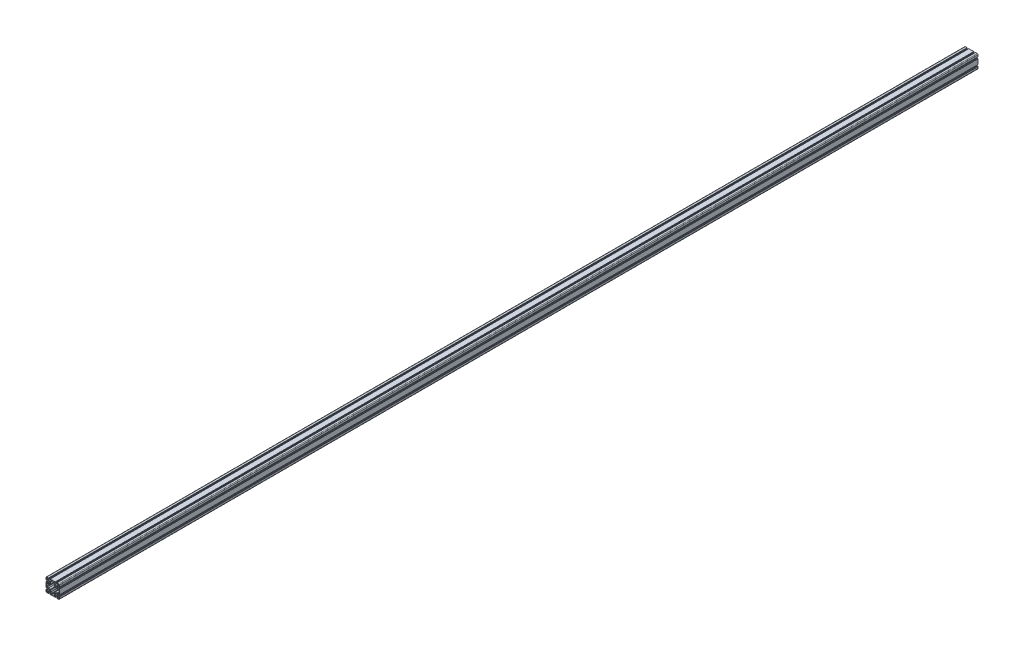
from build123d import *

# Parameters (mm, degrees)
SKETCH1_R           = 3.4
BOSS_EXTRUDE1_DEPTH = 5500


with BuildPart() as part:
    # Sketch1 → Boss-Extrude1 (new body)
    with BuildSketch(Plane.XY.offset(100)):
        with BuildLine():
            Line((37.78472507, 10.370402299), (32.802492023, 10.370402299))
            Line((32.802492023, 10.370402299), (28.48472507, 14.688169252))
            Line((28.48472507, 14.688169252), (28.48472507, 26.552635346))
            Line((28.48472507, 26.552635346), (32.802492023, 30.870402299))
            Line((32.802492023, 30.870402299), (37.78472507, 30.870402299))
            ThreePointArc((37.78472507, 30.870402299), (38.491831851, 30.57750908), (38.78472507, 29.870402299))
            Line((38.78472507, 29.870402299), (38.78472507, 28.220402299))
            ThreePointArc((38.78472507, 28.220402299), (38.491831851, 27.513295518), (37.78472507, 27.220402299))
            Line((37.78472507, 27.220402299), (36.28472507, 27.220402299))
            Line((36.28472507, 27.220402299), (36.28472507, 25.020402299))
            ThreePointArc((36.28472507, 25.020402299), (36.372593036, 24.808270264), (36.58472507, 24.720402299))
            Line((36.58472507, 24.720402299), (39.78472507, 24.720402299))
            Line((39.78472507, 24.720402299), (39.78472507, 25.520402299))
            ThreePointArc((39.78472507, 25.520402299), (39.843303714, 25.661823655), (39.98472507, 25.720402299))
            Line((39.98472507, 25.720402299), (40.78472507, 25.720402299))
            Line((40.78472507, 25.720402299), (40.78472507, 36.120402299))
            ThreePointArc((40.78472507, 36.120402299), (39.466705585, 39.302382814), (36.28472507, 40.620402299))
            Line((36.28472507, 40.620402299), (25.88472507, 40.620402299))
            Line((25.88472507, 40.620402299), (25.88472507, 39.820402299))
            ThreePointArc((25.88472507, 39.820402299), (25.826146426, 39.678980943), (25.68472507, 39.620402299))
            Line((25.68472507, 39.620402299), (24.88472507, 39.620402299))
            Line((24.88472507, 39.620402299), (24.88472507, 36.420402299))
            ThreePointArc((24.88472507, 36.420402299), (24.972593036, 36.208270264), (25.18472507, 36.120402299))
            Line((25.18472507, 36.120402299), (27.38472507, 36.120402299))
            Line((27.38472507, 36.120402299), (27.38472507, 37.620402299))
            ThreePointArc((27.38472507, 37.620402299), (27.677618289, 38.32750908), (28.38472507, 38.620402299))
            Line((28.38472507, 38.620402299), (30.03472507, 38.620402299))
            ThreePointArc((30.03472507, 38.620402299), (30.741831851, 38.32750908), (31.03472507, 37.620402299))
            Line((31.03472507, 37.620402299), (31.03472507, 32.638169252))
            Line((31.03472507, 32.638169252), (26.716958117, 28.320402299))
            Line((26.716958117, 28.320402299), (14.852492023, 28.320402299))
            Line((14.852492023, 28.320402299), (10.53472507, 32.638169252))
            Line((10.53472507, 32.638169252), (10.53472507, 37.620402299))
            ThreePointArc((10.53472507, 37.620402299), (10.827618289, 38.32750908), (11.53472507, 38.620402299))
            Line((11.53472507, 38.620402299), (13.18472507, 38.620402299))
            ThreePointArc((13.18472507, 38.620402299), (13.891831851, 38.32750908), (14.18472507, 37.620402299))
            Line((14.18472507, 37.620402299), (14.18472507, 36.120402299))
            Line((14.18472507, 36.120402299), (16.38472507, 36.120402299))
            ThreePointArc((16.38472507, 36.120402299), (16.596857104, 36.208270264), (16.68472507, 36.420402299))
            Line((16.68472507, 36.420402299), (16.68472507, 39.620402299))
            Line((16.68472507, 39.620402299), (15.88472507, 39.620402299))
            ThreePointArc((15.88472507, 39.620402299), (15.743303714, 39.678980943), (15.68472507, 39.820402299))
            Line((15.68472507, 39.820402299), (15.68472507, 40.620402299))
            Line((15.68472507, 40.620402299), (-14.11527493, 40.620402299))
            Line((-14.11527493, 40.620402299), (-14.11527493, 39.820402299))
            ThreePointArc((-14.11527493, 39.820402299), (-14.173853574, 39.678980943), (-14.31527493, 39.620402299))
            Line((-14.31527493, 39.620402299), (-15.11527493, 39.620402299))
            Line((-15.11527493, 39.620402299), (-15.11527493, 36.420402299))
            ThreePointArc((-15.11527493, 36.420402299), (-15.027406964, 36.208270264), (-14.81527493, 36.120402299))
            Line((-14.81527493, 36.120402299), (-12.61527493, 36.120402299))
            Line((-12.61527493, 36.120402299), (-12.61527493, 37.620402299))
            ThreePointArc((-12.61527493, 37.620402299), (-12.322381711, 38.32750908), (-11.61527493, 38.620402299))
            Line((-11.61527493, 38.620402299), (-9.96527493, 38.620402299))
            ThreePointArc((-9.96527493, 38.620402299), (-9.258168149, 38.32750908), (-8.96527493, 37.620402299))
            Line((-8.96527493, 37.620402299), (-8.96527493, 32.638169252))
            Line((-8.96527493, 32.638169252), (-13.283041883, 28.320402299))
            Line((-13.283041883, 28.320402299), (-25.147507977, 28.320402299))
            Line((-25.147507977, 28.320402299), (-29.46527493, 32.638169252))
            Line((-29.46527493, 32.638169252), (-29.46527493, 37.620402299))
            ThreePointArc((-29.46527493, 37.620402299), (-29.172381711, 38.32750908), (-28.46527493, 38.620402299))
            Line((-28.46527493, 38.620402299), (-26.81527493, 38.620402299))
            ThreePointArc((-26.81527493, 38.620402299), (-26.108168149, 38.32750908), (-25.81527493, 37.620402299))
            Line((-25.81527493, 37.620402299), (-25.81527493, 36.120402299))
            Line((-25.81527493, 36.120402299), (-23.61527493, 36.120402299))
            ThreePointArc((-23.61527493, 36.120402299), (-23.403142896, 36.208270264), (-23.31527493, 36.420402299))
            Line((-23.31527493, 36.420402299), (-23.31527493, 39.620402299))
            Line((-23.31527493, 39.620402299), (-24.11527493, 39.620402299))
            ThreePointArc((-24.11527493, 39.620402299), (-24.256696286, 39.678980943), (-24.31527493, 39.820402299))
            Line((-24.31527493, 39.820402299), (-24.31527493, 40.620402299))
            Line((-24.31527493, 40.620402299), (-34.71527493, 40.620402299))
            ThreePointArc((-34.71527493, 40.620402299), (-37.897255445, 39.302382814), (-39.21527493, 36.120402299))
            Line((-39.21527493, 36.120402299), (-39.21527493, 25.720402299))
            Line((-39.21527493, 25.720402299), (-38.41527493, 25.720402299))
            ThreePointArc((-38.41527493, 25.720402299), (-38.273853574, 25.661823655), (-38.21527493, 25.520402299))
            Line((-38.21527493, 25.520402299), (-38.21527493, 24.720402299))
            Line((-38.21527493, 24.720402299), (-35.01527493, 24.720402299))
            ThreePointArc((-35.01527493, 24.720402299), (-34.803142896, 24.808270264), (-34.71527493, 25.020402299))
            Line((-34.71527493, 25.020402299), (-34.71527493, 27.220402299))
            Line((-34.71527493, 27.220402299), (-36.21527493, 27.220402299))
            ThreePointArc((-36.21527493, 27.220402299), (-36.922381711, 27.513295518), (-37.21527493, 28.220402299))
            Line((-37.21527493, 28.220402299), (-37.21527493, 29.870402299))
            ThreePointArc((-37.21527493, 29.870402299), (-36.922381711, 30.57750908), (-36.21527493, 30.870402299))
            Line((-36.21527493, 30.870402299), (-31.233041883, 30.870402299))
            Line((-31.233041883, 30.870402299), (-26.91527493, 26.552635346))
            Line((-26.91527493, 26.552635346), (-26.91527493, 14.688169252))
            Line((-26.91527493, 14.688169252), (-31.233041883, 10.370402299))
            Line((-31.233041883, 10.370402299), (-36.21527493, 10.370402299))
            ThreePointArc((-36.21527493, 10.370402299), (-36.922381711, 10.663295518), (-37.21527493, 11.370402299))
            Line((-37.21527493, 11.370402299), (-37.21527493, 13.020402299))
            ThreePointArc((-37.21527493, 13.020402299), (-36.922381711, 13.72750908), (-36.21527493, 14.020402299))
            Line((-36.21527493, 14.020402299), (-34.71527493, 14.020402299))
            Line((-34.71527493, 14.020402299), (-34.71527493, 16.220402299))
            ThreePointArc((-34.71527493, 16.220402299), (-34.803142896, 16.432534333), (-35.01527493, 16.520402299))
            Line((-35.01527493, 16.520402299), (-38.21527493, 16.520402299))
            Line((-38.21527493, 16.520402299), (-38.21527493, 15.720402299))
            ThreePointArc((-38.21527493, 15.720402299), (-38.273853574, 15.578980943), (-38.41527493, 15.520402299))
            Line((-38.41527493, 15.520402299), (-39.21527493, 15.520402299))
            Line((-39.21527493, 15.520402299), (-39.21527493, -14.279597701))
            Line((-39.21527493, -14.279597701), (-38.41527493, -14.279597701))
            ThreePointArc((-38.41527493, -14.279597701), (-38.273853574, -14.338176345), (-38.21527493, -14.479597701))
            Line((-38.21527493, -14.479597701), (-38.21527493, -15.279597701))
            Line((-38.21527493, -15.279597701), (-35.01527493, -15.279597701))
            ThreePointArc((-35.01527493, -15.279597701), (-34.803142896, -15.191729736), (-34.71527493, -14.979597701))
            Line((-34.71527493, -14.979597701), (-34.71527493, -12.779597701))
            Line((-34.71527493, -12.779597701), (-36.21527493, -12.779597701))
            ThreePointArc((-36.21527493, -12.779597701), (-36.922381711, -12.486704482), (-37.21527493, -11.779597701))
            Line((-37.21527493, -11.779597701), (-37.21527493, -10.129597701))
            ThreePointArc((-37.21527493, -10.129597701), (-36.922381711, -9.42249092), (-36.21527493, -9.129597701))
            Line((-36.21527493, -9.129597701), (-31.233041883, -9.129597701))
            Line((-31.233041883, -9.129597701), (-26.91527493, -13.447364654))
            Line((-26.91527493, -13.447364654), (-26.91527493, -25.311830748))
            Line((-26.91527493, -25.311830748), (-31.233041883, -29.629597701))
            Line((-31.233041883, -29.629597701), (-36.21527493, -29.629597701))
            ThreePointArc((-36.21527493, -29.629597701), (-36.922381711, -29.336704482), (-37.21527493, -28.629597701))
            Line((-37.21527493, -28.629597701), (-37.21527493, -26.979597701))
            ThreePointArc((-37.21527493, -26.979597701), (-36.922381711, -26.27249092), (-36.21527493, -25.979597701))
            Line((-36.21527493, -25.979597701), (-34.71527493, -25.979597701))
            Line((-34.71527493, -25.979597701), (-34.71527493, -23.779597701))
            ThreePointArc((-34.71527493, -23.779597701), (-34.803142896, -23.567465667), (-35.01527493, -23.479597701))
            Line((-35.01527493, -23.479597701), (-38.21527493, -23.479597701))
            Line((-38.21527493, -23.479597701), (-38.21527493, -24.279597701))
            ThreePointArc((-38.21527493, -24.279597701), (-38.273853574, -24.421019057), (-38.41527493, -24.479597701))
            Line((-38.41527493, -24.479597701), (-39.21527493, -24.479597701))
            Line((-39.21527493, -24.479597701), (-39.21527493, -34.879597701))
            ThreePointArc((-39.21527493, -34.879597701), (-37.897255445, -38.061578216), (-34.71527493, -39.379597701))
            Line((-34.71527493, -39.379597701), (-24.31527493, -39.379597701))
            Line((-24.31527493, -39.379597701), (-24.31527493, -38.579597701))
            ThreePointArc((-24.31527493, -38.579597701), (-24.256696286, -38.438176345), (-24.11527493, -38.379597701))
            Line((-24.11527493, -38.379597701), (-23.31527493, -38.379597701))
            Line((-23.31527493, -38.379597701), (-23.31527493, -35.179597701))
            ThreePointArc((-23.31527493, -35.179597701), (-23.403142896, -34.967465667), (-23.61527493, -34.879597701))
            Line((-23.61527493, -34.879597701), (-25.81527493, -34.879597701))
            Line((-25.81527493, -34.879597701), (-25.81527493, -36.379597701))
            ThreePointArc((-25.81527493, -36.379597701), (-26.108168149, -37.086704482), (-26.81527493, -37.379597701))
            Line((-26.81527493, -37.379597701), (-28.46527493, -37.379597701))
            ThreePointArc((-28.46527493, -37.379597701), (-29.172381711, -37.086704482), (-29.46527493, -36.379597701))
            Line((-29.46527493, -36.379597701), (-29.46527493, -31.397364654))
            Line((-29.46527493, -31.397364654), (-25.147507977, -27.079597701))
            Line((-25.147507977, -27.079597701), (-13.283041883, -27.079597701))
            Line((-13.283041883, -27.079597701), (-8.96527493, -31.397364654))
            Line((-8.96527493, -31.397364654), (-8.96527493, -36.379597701))
            ThreePointArc((-8.96527493, -36.379597701), (-9.258168149, -37.086704482), (-9.96527493, -37.379597701))
            Line((-9.96527493, -37.379597701), (-11.61527493, -37.379597701))
            ThreePointArc((-11.61527493, -37.379597701), (-12.322381711, -37.086704482), (-12.61527493, -36.379597701))
            Line((-12.61527493, -36.379597701), (-12.61527493, -34.879597701))
            Line((-12.61527493, -34.879597701), (-14.81527493, -34.879597701))
            ThreePointArc((-14.81527493, -34.879597701), (-15.027406964, -34.967465667), (-15.11527493, -35.179597701))
            Line((-15.11527493, -35.179597701), (-15.11527493, -38.379597701))
            Line((-15.11527493, -38.379597701), (-14.31527493, -38.379597701))
            ThreePointArc((-14.31527493, -38.379597701), (-14.173853574, -38.438176345), (-14.11527493, -38.579597701))
            Line((-14.11527493, -38.579597701), (-14.11527493, -39.379597701))
            Line((-14.11527493, -39.379597701), (15.68472507, -39.379597701))
            Line((15.68472507, -39.379597701), (15.68472507, -38.579597701))
            ThreePointArc((15.68472507, -38.579597701), (15.743303714, -38.438176345), (15.88472507, -38.379597701))
            Line((15.88472507, -38.379597701), (16.68472507, -38.379597701))
            Line((16.68472507, -38.379597701), (16.68472507, -35.179597701))
            ThreePointArc((16.68472507, -35.179597701), (16.596857104, -34.967465667), (16.38472507, -34.879597701))
            Line((16.38472507, -34.879597701), (14.18472507, -34.879597701))
            Line((14.18472507, -34.879597701), (14.18472507, -36.379597701))
            ThreePointArc((14.18472507, -36.379597701), (13.891831851, -37.086704482), (13.18472507, -37.379597701))
            Line((13.18472507, -37.379597701), (11.53472507, -37.379597701))
            ThreePointArc((11.53472507, -37.379597701), (10.827618289, -37.086704482), (10.53472507, -36.379597701))
            Line((10.53472507, -36.379597701), (10.53472507, -31.397364654))
            Line((10.53472507, -31.397364654), (14.852492023, -27.079597701))
            Line((14.852492023, -27.079597701), (26.716958117, -27.079597701))
            Line((26.716958117, -27.079597701), (31.03472507, -31.397364654))
            Line((31.03472507, -31.397364654), (31.03472507, -36.379597701))
            ThreePointArc((31.03472507, -36.379597701), (30.741831851, -37.086704482), (30.03472507, -37.379597701))
            Line((30.03472507, -37.379597701), (28.38472507, -37.379597701))
            ThreePointArc((28.38472507, -37.379597701), (27.677618289, -37.086704482), (27.38472507, -36.379597701))
            Line((27.38472507, -36.379597701), (27.38472507, -34.879597701))
            Line((27.38472507, -34.879597701), (25.18472507, -34.879597701))
            ThreePointArc((25.18472507, -34.879597701), (24.972593036, -34.967465667), (24.88472507, -35.179597701))
            Line((24.88472507, -35.179597701), (24.88472507, -38.379597701))
            Line((24.88472507, -38.379597701), (25.68472507, -38.379597701))
            ThreePointArc((25.68472507, -38.379597701), (25.826146426, -38.438176345), (25.88472507, -38.579597701))
            Line((25.88472507, -38.579597701), (25.88472507, -39.379597701))
            Line((25.88472507, -39.379597701), (36.28472507, -39.379597701))
            ThreePointArc((36.28472507, -39.379597701), (39.466705585, -38.061578216), (40.78472507, -34.879597701))
            Line((40.78472507, -34.879597701), (40.78472507, -24.479597701))
            Line((40.78472507, -24.479597701), (39.98472507, -24.479597701))
            ThreePointArc((39.98472507, -24.479597701), (39.843303714, -24.421019057), (39.78472507, -24.279597701))
            Line((39.78472507, -24.279597701), (39.78472507, -23.479597701))
            Line((39.78472507, -23.479597701), (36.58472507, -23.479597701))
            ThreePointArc((36.58472507, -23.479597701), (36.372593036, -23.567465667), (36.28472507, -23.779597701))
            Line((36.28472507, -23.779597701), (36.28472507, -25.979597701))
            Line((36.28472507, -25.979597701), (37.78472507, -25.979597701))
            ThreePointArc((37.78472507, -25.979597701), (38.491831851, -26.27249092), (38.78472507, -26.979597701))
            Line((38.78472507, -26.979597701), (38.78472507, -28.629597701))
            ThreePointArc((38.78472507, -28.629597701), (38.491831851, -29.336704482), (37.78472507, -29.629597701))
            Line((37.78472507, -29.629597701), (32.802492023, -29.629597701))
            Line((32.802492023, -29.629597701), (28.48472507, -25.311830748))
            Line((28.48472507, -25.311830748), (28.48472507, -13.447364654))
            Line((28.48472507, -13.447364654), (32.802492023, -9.129597701))
            Line((32.802492023, -9.129597701), (37.78472507, -9.129597701))
            ThreePointArc((37.78472507, -9.129597701), (38.491831851, -9.42249092), (38.78472507, -10.129597701))
            Line((38.78472507, -10.129597701), (38.78472507, -11.779597701))
            ThreePointArc((38.78472507, -11.779597701), (38.491831851, -12.486704482), (37.78472507, -12.779597701))
            Line((37.78472507, -12.779597701), (36.28472507, -12.779597701))
            Line((36.28472507, -12.779597701), (36.28472507, -14.979597701))
            ThreePointArc((36.28472507, -14.979597701), (36.372593036, -15.191729736), (36.58472507, -15.279597701))
            Line((36.58472507, -15.279597701), (39.78472507, -15.279597701))
            Line((39.78472507, -15.279597701), (39.78472507, -14.479597701))
            ThreePointArc((39.78472507, -14.479597701), (39.843303714, -14.338176345), (39.98472507, -14.279597701))
            Line((39.98472507, -14.279597701), (40.78472507, -14.279597701))
            Line((40.78472507, -14.279597701), (40.78472507, 15.520402299))
            Line((40.78472507, 15.520402299), (39.98472507, 15.520402299))
            ThreePointArc((39.98472507, 15.520402299), (39.843303714, 15.578980943), (39.78472507, 15.720402299))
            Line((39.78472507, 15.720402299), (39.78472507, 16.520402299))
            Line((39.78472507, 16.520402299), (36.58472507, 16.520402299))
            ThreePointArc((36.58472507, 16.520402299), (36.372593036, 16.432534333), (36.28472507, 16.220402299))
            Line((36.28472507, 16.220402299), (36.28472507, 14.020402299))
            Line((36.28472507, 14.020402299), (37.78472507, 14.020402299))
            ThreePointArc((37.78472507, 14.020402299), (38.491831851, 13.72750908), (38.78472507, 13.020402299))
            Line((38.78472507, 13.020402299), (38.78472507, 11.370402299))
            ThreePointArc((38.78472507, 11.370402299), (38.491831851, 10.663295518), (37.78472507, 10.370402299))
        make_face()
        with Locations(Location((-19.21527493, -19.379597701, 0), (0, 0, 180))):
            Circle(SKETCH1_R, mode=Mode.SUBTRACT)
        with Locations(Location((20.78472507, -19.379597701, 0), (0, 0, 180))):
            Circle(SKETCH1_R, mode=Mode.SUBTRACT)
        with Locations(Location((20.78472507, 20.620402299, 0), (0, 0, 180))):
            Circle(SKETCH1_R, mode=Mode.SUBTRACT)
        with Locations(Location((-19.21527493, 20.620402299, 0), (0, 0, 180))):
            Circle(SKETCH1_R, mode=Mode.SUBTRACT)
        with BuildLine():
            Line((-29.61172154, 8.456188736), (-25.147507977, 12.920402299))
            Line((-25.147507977, 12.920402299), (-14.01527493, 12.920402299))
            ThreePointArc((-14.01527493, 12.920402299), (-12.247507977, 13.652635346), (-11.51527493, 15.420402299))
            Line((-11.51527493, 15.420402299), (-11.51527493, 26.552635346))
            Line((-11.51527493, 26.552635346), (-7.051061368, 31.016848908))
            ThreePointArc((-7.051061368, 31.016848908), (-6.617515865, 31.665695606), (-6.46527493, 32.431062471))
            Line((-6.46527493, 32.431062471), (-6.46527493, 37.420402299))
            ThreePointArc((-6.46527493, 37.420402299), (-6.172381711, 38.12750908), (-5.46527493, 38.420402299))
            Line((-5.46527493, 38.420402299), (7.03472507, 38.420402299))
            ThreePointArc((7.03472507, 38.420402299), (7.741831851, 38.12750908), (8.03472507, 37.420402299))
            Line((8.03472507, 37.420402299), (8.03472507, 32.431062471))
            ThreePointArc((8.03472507, 32.431062471), (8.186966005, 31.665695606), (8.620511508, 31.016848908))
            Line((8.620511508, 31.016848908), (13.08472507, 26.552635346))
            Line((13.08472507, 26.552635346), (13.08472507, 15.420402299))
            ThreePointArc((13.08472507, 15.420402299), (13.816958117, 13.652635346), (15.58472507, 12.920402299))
            Line((15.58472507, 12.920402299), (26.716958117, 12.920402299))
            Line((26.716958117, 12.920402299), (31.181171679, 8.456188736))
            ThreePointArc((31.181171679, 8.456188736), (31.830018377, 8.022643234), (32.595385242, 7.870402299))
            Line((32.595385242, 7.870402299), (37.58472507, 7.870402299))
            ThreePointArc((37.58472507, 7.870402299), (38.291831851, 7.57750908), (38.58472507, 6.870402299))
            Line((38.58472507, 6.870402299), (38.58472507, -5.629597701))
            ThreePointArc((38.58472507, -5.629597701), (38.291831851, -6.336704482), (37.58472507, -6.629597701))
            Line((37.58472507, -6.629597701), (32.595385242, -6.629597701))
            ThreePointArc((32.595385242, -6.629597701), (31.830018377, -6.781838636), (31.181171679, -7.215384139))
            Line((31.181171679, -7.215384139), (26.716958117, -11.679597701))
            Line((26.716958117, -11.679597701), (15.58472507, -11.679597701))
            ThreePointArc((15.58472507, -11.679597701), (13.816958117, -12.411830748), (13.08472507, -14.179597701))
            Line((13.08472507, -14.179597701), (13.08472507, -24.483403623))
            ThreePointArc((13.08472507, -24.483403623), (12.932484135, -25.248770488), (12.498938632, -25.897617186))
            Line((12.498938632, -25.897617186), (8.620511508, -29.776044311))
            ThreePointArc((8.620511508, -29.776044311), (8.186966005, -30.424891008), (8.03472507, -31.190257873))
            Line((8.03472507, -31.190257873), (8.03472507, -36.179597701))
            ThreePointArc((8.03472507, -36.179597701), (7.741831851, -36.886704482), (7.03472507, -37.179597701))
            Line((7.03472507, -37.179597701), (-5.46527493, -37.179597701))
            ThreePointArc((-5.46527493, -37.179597701), (-6.172381711, -36.886704482), (-6.46527493, -36.179597701))
            Line((-6.46527493, -36.179597701), (-6.46527493, -31.190257873))
            ThreePointArc((-6.46527493, -31.190257873), (-6.617515865, -30.424891008), (-7.051061368, -29.776044311))
            Line((-7.051061368, -29.776044311), (-11.51527493, -25.311830748))
            Line((-11.51527493, -25.311830748), (-11.51527493, -14.179597701))
            ThreePointArc((-11.51527493, -14.179597701), (-12.247507977, -12.411830748), (-14.01527493, -11.679597701))
            Line((-14.01527493, -11.679597701), (-25.147507977, -11.679597701))
            Line((-25.147507977, -11.679597701), (-29.61172154, -7.215384139))
            ThreePointArc((-29.61172154, -7.215384139), (-30.260568237, -6.781838636), (-31.025935102, -6.629597701))
            Line((-31.025935102, -6.629597701), (-36.01527493, -6.629597701))
            ThreePointArc((-36.01527493, -6.629597701), (-36.722381711, -6.336704482), (-37.01527493, -5.629597701))
            Line((-37.01527493, -5.629597701), (-37.01527493, 6.870402299))
            ThreePointArc((-37.01527493, 6.870402299), (-36.722381711, 7.57750908), (-36.01527493, 7.870402299))
            Line((-36.01527493, 7.870402299), (-31.025935102, 7.870402299))
            ThreePointArc((-31.025935102, 7.870402299), (-30.260568237, 8.022643234), (-29.61172154, 8.456188736))
        make_face(mode=Mode.SUBTRACT)
        with BuildLine():
            Line((-35.21927493, 39.124402299), (-31.96527493, 39.124402299))
            ThreePointArc((-31.96527493, 39.124402299), (-31.258168149, 38.83150908), (-30.96527493, 38.124402299))
            Line((-30.96527493, 38.124402299), (-30.96527493, 33.370402299))
            ThreePointArc((-30.96527493, 33.370402299), (-31.258168149, 32.663295518), (-31.96527493, 32.370402299))
            Line((-31.96527493, 32.370402299), (-36.71927493, 32.370402299))
            ThreePointArc((-36.71927493, 32.370402299), (-37.426381711, 32.663295518), (-37.71927493, 33.370402299))
            Line((-37.71927493, 33.370402299), (-37.71927493, 36.624402299))
            ThreePointArc((-37.71927493, 36.624402299), (-36.987041883, 38.392169252), (-35.21927493, 39.124402299))
        make_face(mode=Mode.SUBTRACT)
        with BuildLine():
            Line((36.78872507, -37.883597701), (33.53472507, -37.883597701))
            ThreePointArc((33.53472507, -37.883597701), (32.827618289, -37.590704482), (32.53472507, -36.883597701))
            Line((32.53472507, -36.883597701), (32.53472507, -32.129597701))
            ThreePointArc((32.53472507, -32.129597701), (32.827618289, -31.42249092), (33.53472507, -31.129597701))
            Line((33.53472507, -31.129597701), (38.28872507, -31.129597701))
            ThreePointArc((38.28872507, -31.129597701), (38.995831851, -31.42249092), (39.28872507, -32.129597701))
            Line((39.28872507, -32.129597701), (39.28872507, -35.383597701))
            ThreePointArc((39.28872507, -35.383597701), (38.556492023, -37.151364654), (36.78872507, -37.883597701))
        make_face(mode=Mode.SUBTRACT)
        with BuildLine():
            Line((-37.71927493, -35.383597701), (-37.71927493, -32.129597701))
            ThreePointArc((-37.71927493, -32.129597701), (-37.426381711, -31.42249092), (-36.71927493, -31.129597701))
            Line((-36.71927493, -31.129597701), (-31.96527493, -31.129597701))
            ThreePointArc((-31.96527493, -31.129597701), (-31.258168149, -31.42249092), (-30.96527493, -32.129597701))
            Line((-30.96527493, -32.129597701), (-30.96527493, -36.883597701))
            ThreePointArc((-30.96527493, -36.883597701), (-31.258168149, -37.590704482), (-31.96527493, -37.883597701))
            Line((-31.96527493, -37.883597701), (-35.21927493, -37.883597701))
            ThreePointArc((-35.21927493, -37.883597701), (-36.987041883, -37.151364654), (-37.71927493, -35.383597701))
        make_face(mode=Mode.SUBTRACT)
        with BuildLine():
            Line((39.28872507, 36.624402299), (39.28872507, 33.370402299))
            ThreePointArc((39.28872507, 33.370402299), (38.995831851, 32.663295518), (38.28872507, 32.370402299))
            Line((38.28872507, 32.370402299), (33.53472507, 32.370402299))
            ThreePointArc((33.53472507, 32.370402299), (32.827618289, 32.663295518), (32.53472507, 33.370402299))
            Line((32.53472507, 33.370402299), (32.53472507, 38.124402299))
            ThreePointArc((32.53472507, 38.124402299), (32.827618289, 38.83150908), (33.53472507, 39.124402299))
            Line((33.53472507, 39.124402299), (36.78872507, 39.124402299))
            ThreePointArc((36.78872507, 39.124402299), (38.556492023, 38.392169252), (39.28872507, 36.624402299))
        make_face(mode=Mode.SUBTRACT)
    extrude(amount=-BOSS_EXTRUDE1_DEPTH)


solid = part.part
